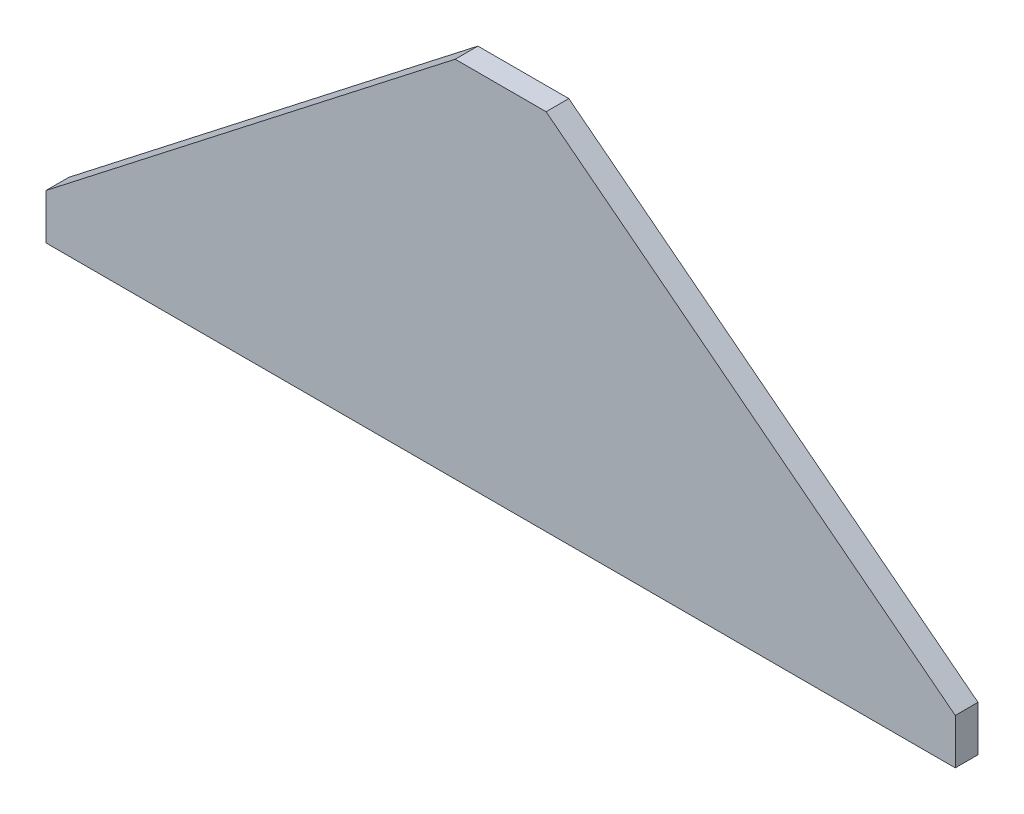
from build123d import *

# Parameters (mm, degrees)
EXTRUDE_1_DEPTH = 5


with BuildPart() as part:
    # 草图1 → 凸台-拉伸1 (new body)
    with BuildSketch(Plane.XY):
        Polygon((-10, 20.230052867), (-100, -49.769947133), (-100, -59.769947133), (100, -59.769947133), (100, -49.769947133), (10, 20.230052867), align=None)
    extrude(amount=EXTRUDE_1_DEPTH)


solid = part.part
